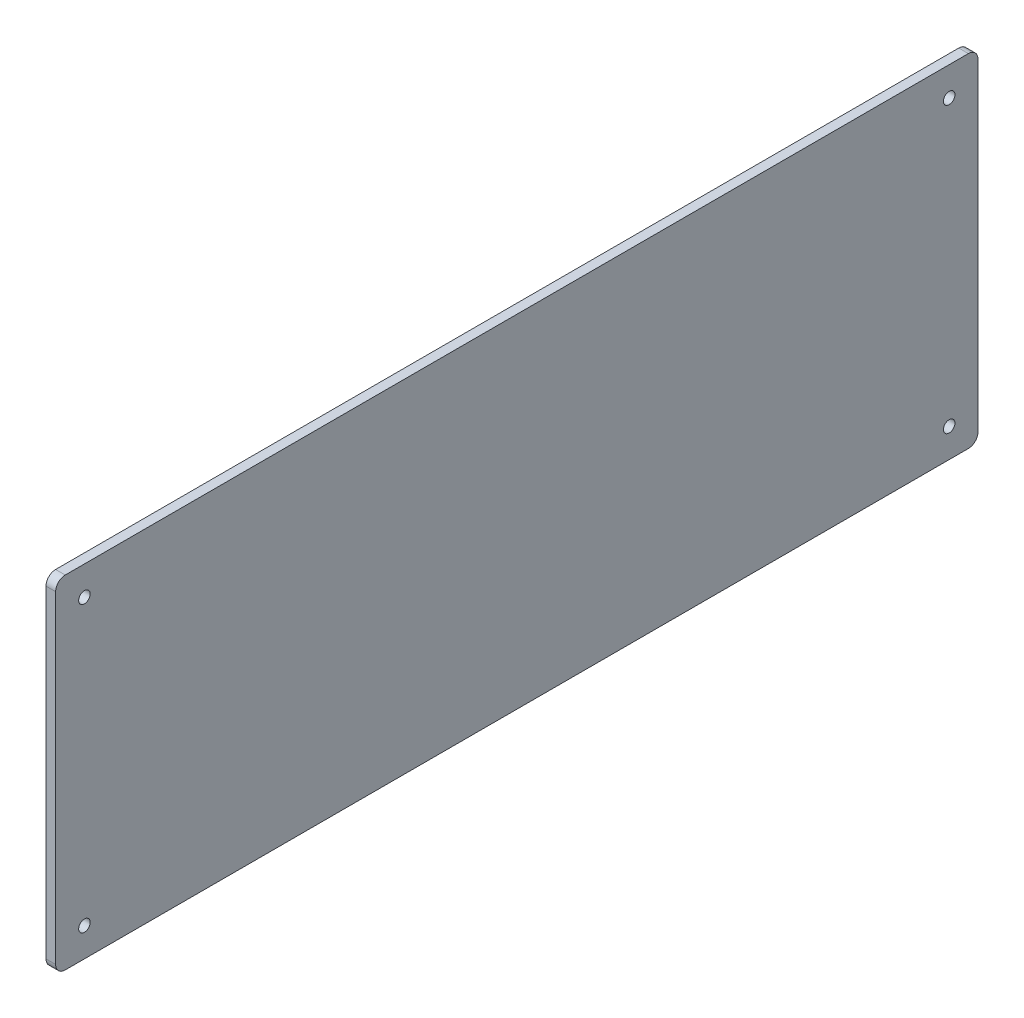
SolidWorks part; units mm, degrees
ref_plane "前视基准面" through (0, 0, 0) normal (0, 0, 1) x (1, 0, 0)
ref_plane "上视基准面" through (0, 0, 0) normal (0, 1, 0) x (1, 0, 0)
ref_plane "右视基准面" through (0, 0, 0) normal (1, 0, 0) x (0, 0, -1)
sketch "草图1" plane through (0, 0, 0) normal (1, 0, 0) x (0, 0, -1)
  line L0 (0, 89) -> (0, 0) construction
  line L1 (-240, 89) -> (240, 89)
  line L2 (-240, 89) -> (-240, -89)
  line L3 (-240, -89) -> (240, -89)
  line L4 (240, 89) -> (240, -89)
  line L5 (0, 0) -> (240, 0) construction
  dimension "D1" = 480
  dimension "D2" = 178
extrude "凸台-拉伸1" add sketch "草图1" along normal blind 5
sketch "草图2" plane through (5, 0, 0) normal (1, 0, 0) x (0, 0, -1)
  line L0 (0, 131.9543) -> (0, 0) construction
  line L1 (0, 0) -> (347.0268, 0) construction
  circle A0 centre (-225, 74) radius 3
  circle A1 centre (225, 74) radius 3
  circle A2 centre (-225, -74) radius 3
  circle A3 centre (225, -74) radius 3
  dimension "D1" = 6
  dimension "D2" = 450
  dimension "D3" = 148
extrude "切除-拉伸1" cut sketch "草图2" against normal through all
fillet "圆角1" radius 5 4 edges at (2.5, -89, 240) (2.5, -89, -240) (2.5, 89, -240) (2.5, 89, 240)
